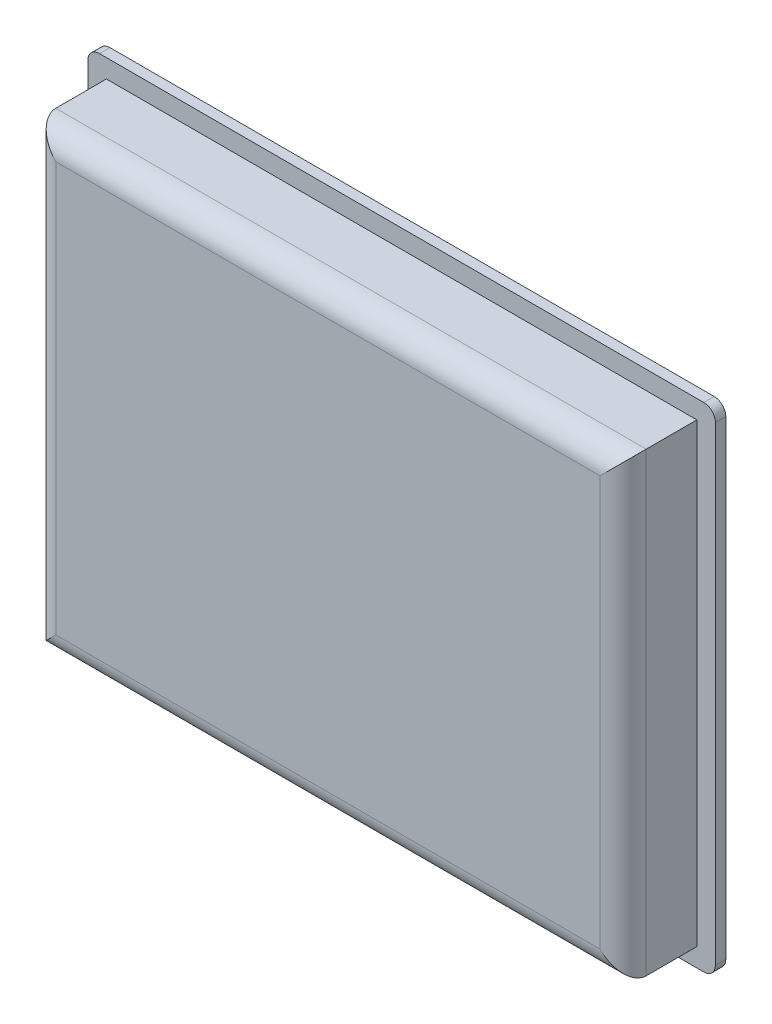
from build123d import *

# Parameters (mm, degrees)
SKETCH_1_W          = 271
SKETCH_1_H          = 213
EXTRUDE_1_DEPTH     = 4.5
SKETCH_2_W          = 255
SKETCH_2_H          = 197
EXTRUDE_2_DEPTH     = 31.86
FILLET_1_R          = 10
FILLET_2_R          = 5
SKETCH_4_W          = 220
SKETCH_4_H          = 140
CUT_EXTRUDE_1_DEPTH = 3


with BuildPart() as part:
    # 草图1 → 凸台-拉伸1 (new body)
    with BuildSketch(Plane.XY):
        with Locations((135.5, -106.5)):
            Rectangle(SKETCH_1_W, SKETCH_1_H)
    extrude(amount=EXTRUDE_1_DEPTH)

    # 草图2 → 凸台-拉伸2 (add)
    with BuildSketch(Plane.XY.offset(4.5)):
        with Locations((135.5, -106.5)):
            Rectangle(SKETCH_2_W, SKETCH_2_H)
    extrude(amount=EXTRUDE_2_DEPTH)

    # 圆角1
    fillet_1_edges = [part.edges().sort_by_distance(p)[0] for p in [
        (263, -106.5, 36.36),
        (135.5, -8, 36.36),
        (8, -106.5, 36.36),
        (135.5, -205, 36.36),
    ]]
    fillet(fillet_1_edges, radius=FILLET_1_R)

    # 圆角2
    fillet_2_edges = [part.edges().sort_by_distance(p)[0] for p in [
        (0, 0, 2.25),
        (271, 0, 2.25),
        (271, -213, 2.25),
        (0, -213, 2.25),
    ]]
    fillet(fillet_2_edges, radius=FILLET_2_R)

    # 草图4 → 切除-拉伸1 (cut)
    with BuildSketch(Plane(origin=(0, 0, 0), x_dir=(-1, 0, 0), z_dir=(0, 0, -1))):
        with Locations((-135.5, -106.5)):
            Rectangle(SKETCH_4_W, SKETCH_4_H)
    extrude(amount=-CUT_EXTRUDE_1_DEPTH, mode=Mode.SUBTRACT)


solid = part.part
